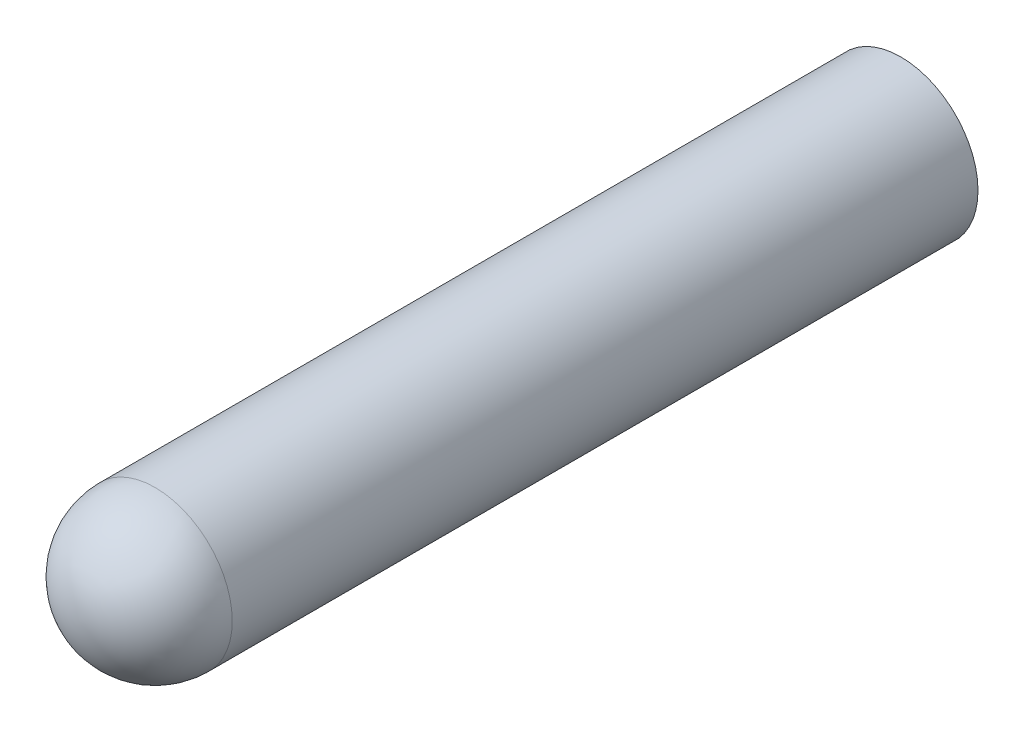
SolidWorks part; units mm, degrees
ref_plane "Front Plane" through (0, 0, 0) normal (0, 0, 1) x (1, 0, 0)
ref_plane "Top Plane" through (0, 0, 0) normal (0, 1, 0) x (1, 0, 0)
ref_plane "Right Plane" through (0, 0, 0) normal (1, 0, 0) x (0, 0, -1)
other "Configuration Table"
sketch "Sketch1" plane through (0, 0, 0) normal (0, 0, 1) x (1, 0, 0)
  circle A0 centre (0, 0) radius 1.5
  dimension "D1" = 3
extrude "Boss-Extrude1" add sketch "Sketch1" along normal blind 16
fillet "Fillet1" radius 1.5 1 edges at (1.5, 0, 16)
